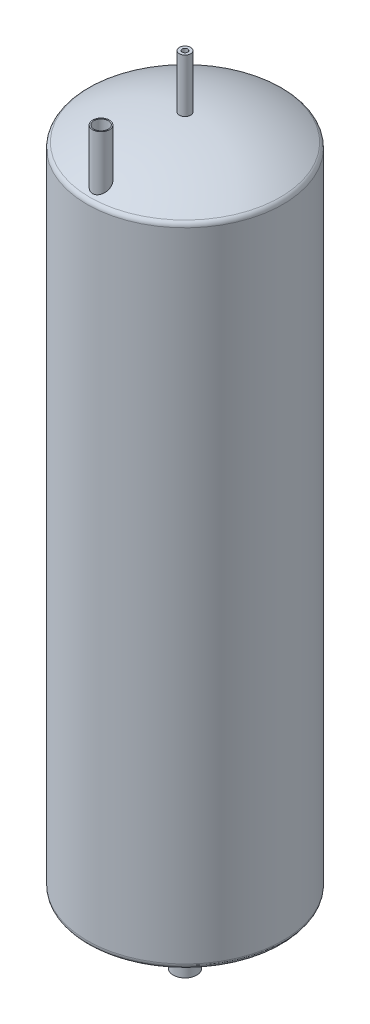
from build123d import *

# Parameters (mm, degrees)
BOSS_EXTRUDE1_REACH      = 1349.915
BOSS_EXTRUDE1_END_RADIUS = 331.651906797
SKETCH2_R                = 21
SKETCH2_R_2              = 18.5
SKETCH3_R                = 18.5
CUT_EXTRUDE1_DEPTH       = 526
BOSS_EXTRUDE3_REACH      = 1443.406
BOSS_EXTRUDE3_END_RADIUS = 331.651906797
SKETCH5_R                = 10
SKETCH5_R_2              = 5
SKETCH6_R                = 5
CUT_EXTRUDE2_DEPTH       = 190
BOSS_EXTRUDE5_REACH      = 1404.016
BOSS_EXTRUDE5_END_RADIUS = 331.651906797
SKETCH8_R                = 15
SKETCH8_R_2              = 13
SKETCH9_R                = 13.000001432
CUT_EXTRUDE3_DEPTH       = 107


with BuildPart() as part:
    # Sketch1 → Revolve1 (revolve)
    with BuildSketch(Plane.XY, mode=Mode.PRIVATE) as revolve1_sk:
        with BuildLine():
            Line((175, -569.454864482), (175, 569.454864482))
            ThreePointArc((175, 569.454864482), (173.697634466, 574.389553398), (170.129769061, 578.03888856))
            ThreePointArc((170.129769061, 578.03888856), (88.246082503, 613.044224248), (0, 625))
            Line((0, 625), (0, 620))
            ThreePointArc((0, 620), (85.508108026, 608.609622217), (165.052867094, 575.232855612))
            ThreePointArc((165.052867094, 575.232855612), (168.67550203, 571.57683653), (170, 566.603340322))
            Line((170, 566.603340322), (170, -566.603340322))
            ThreePointArc((170, -566.603340322), (168.67550203, -571.57683653), (165.052867094, -575.232855612))
            ThreePointArc((165.052867094, -575.232855612), (85.508108026, -608.609622217), (0, -620))
            Line((0, -620), (0, -625))
            ThreePointArc((0, -625), (88.246082503, -613.044224248), (170.129769061, -578.03888856))
            ThreePointArc((170.129769061, -578.03888856), (173.697634466, -574.389553398), (175, -569.454864482))
        make_face()
    revolve(revolve1_sk.sketch.rotate(Axis((0, 0, 0), (0, 1, 0)), 90), axis=Axis((0, 0, 0), (0, 1, 0)))

    # Boss-Extrude1: up to this sphere (the profile starts outside it)
    boss_extrude1_end = Location((0, -293.348093203, 0)) * Sphere(BOSS_EXTRUDE1_END_RADIUS, mode=Mode.PRIVATE)
    # Sketch2 → Boss-Extrude1 (add, up to the surface)
    with BuildSketch(Plane(origin=(0, -700, 0), x_dir=(1, 0, 0), z_dir=(0, 1, 0)), mode=Mode.PRIVATE) as boss_extrude1_sk1:
        with Locations(Location((0, 0, 0), (0, 0, 180))):
            Circle(SKETCH2_R)
        with Locations(Location((0, 0, 0), (0, 0, 270))):
            Circle(SKETCH2_R_2, mode=Mode.SUBTRACT)
    boss_extrude1_tool1 = extrude(boss_extrude1_sk1.sketch, amount=BOSS_EXTRUDE1_REACH, mode=Mode.PRIVATE) - boss_extrude1_end
    add(boss_extrude1_tool1.solids().sort_by_distance((20.40603, -700, 0))[0])

    # Sketch3 → Cut-Extrude1 (cut)
    with BuildSketch(Plane(origin=(0, -700, 0), x_dir=(1, 0, 0), z_dir=(0, 1, 0))):
        Circle(SKETCH3_R)
    extrude(amount=CUT_EXTRUDE1_DEPTH, mode=Mode.SUBTRACT)

    # Boss-Extrude3: up to this sphere (the profile starts outside it)
    boss_extrude3_end = Location((0, 293.348093203, 0)) * Sphere(BOSS_EXTRUDE3_END_RADIUS, mode=Mode.PRIVATE)
    # Sketch5 → Boss-Extrude3 (add, up to the surface)
    with BuildSketch(Plane(origin=(0, 720, 0), x_dir=(1, 0, 0), z_dir=(0, 1, 0)), mode=Mode.PRIVATE) as boss_extrude3_sk1:
        with Locations(Location((0, 0, 0), (0, 0, 270))):
            Circle(SKETCH5_R)
        with Locations(Location((0, 0, 0), (0, 0, 270))):
            Circle(SKETCH5_R_2, mode=Mode.SUBTRACT)
    boss_extrude3_tool1 = extrude(boss_extrude3_sk1.sketch, amount=-BOSS_EXTRUDE3_REACH, mode=Mode.PRIVATE) - boss_extrude3_end
    add(boss_extrude3_tool1.solids().sort_by_distance((0, 720, -9.717157))[0])

    # Sketch6 → Cut-Extrude2 (cut)
    with BuildSketch(Plane(origin=(0, 720, 0), x_dir=(1, 0, 0), z_dir=(0, 1, 0))):
        with Locations(Location((0, 0, 0), (0, 0, 270))):
            Circle(SKETCH6_R)
    extrude(amount=-CUT_EXTRUDE2_DEPTH, mode=Mode.SUBTRACT)

    # Boss-Extrude5: up to this sphere (the profile starts outside it)
    boss_extrude5_end = Location((0, 293.348093203, 0)) * Sphere(BOSS_EXTRUDE5_END_RADIUS, mode=Mode.PRIVATE)
    # Sketch8 → Boss-Extrude5 (add, up to the surface)
    with BuildSketch(Plane(origin=(0, 680, 0), x_dir=(1, 0, 0), z_dir=(0, 1, 0)), mode=Mode.PRIVATE) as boss_extrude5_sk1:
        with Locations(Location((0, -150, 0), (0, 0, 270.000000007))):
            Circle(SKETCH8_R)
        with Locations(Location((0, -150, 0), (0, 0, 270))):
            Circle(SKETCH8_R_2, mode=Mode.SUBTRACT)
    boss_extrude5_tool1 = extrude(boss_extrude5_sk1.sketch, amount=-BOSS_EXTRUDE5_REACH, mode=Mode.PRIVATE) - boss_extrude5_end
    add(boss_extrude5_tool1.solids().sort_by_distance((0, 680, 135.424264))[0])

    # Sketch9 → Cut-Extrude3 (cut)
    with BuildSketch(Plane(origin=(0, 680, 0), x_dir=(1, 0, 0), z_dir=(0, 1, 0))):
        with Locations(Location((0, -150, 0), (0, 0, 270))):
            Circle(SKETCH9_R)
    extrude(amount=-CUT_EXTRUDE3_DEPTH, mode=Mode.SUBTRACT)


solid = part.part
